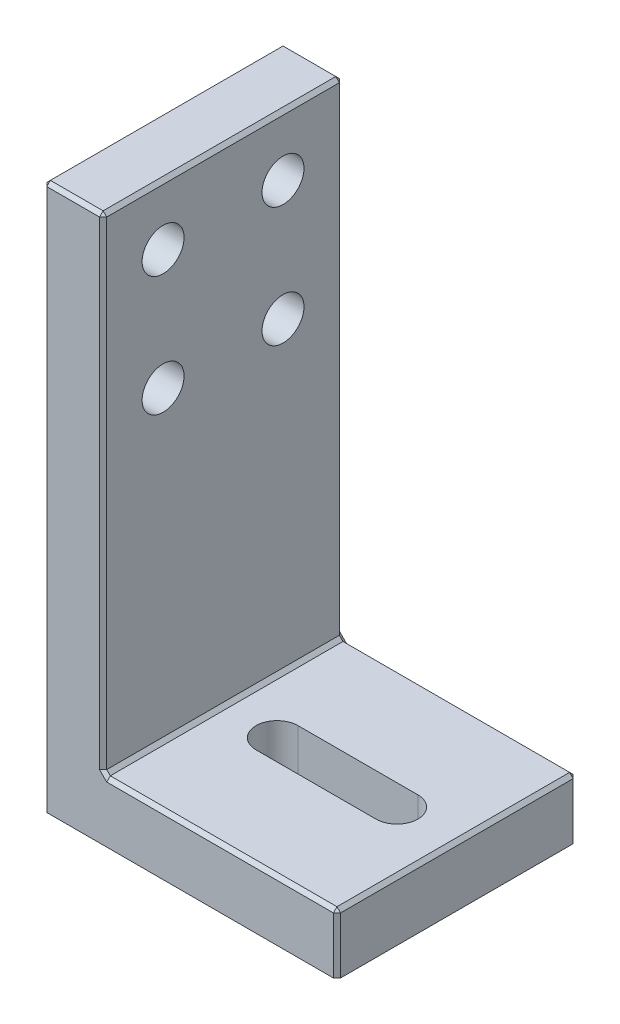
from build123d import *

# Parameters (mm, degrees)
EXTRUDE_THIN1_DEPTH = 20
CHAMFER1_SIZE       = 0.3
CUT_EXTRUDE1_REACH  = 53.386
CUT_EXTRUDE2_REACH  = 55.39
SKETCH3_R           = 1.75


with BuildPart() as part:
    # Sketch1 → Extrude-Thin1 (new body)
    with BuildSketch(Plane.XY):
        Polygon((0, 45.5), (0, 0), (24.5, 0), (24.5, 5), (5, 5), (5, 45.5), align=None)
    extrude(amount=EXTRUDE_THIN1_DEPTH)

    # Chamfer1
    chamfer1_edges = [part.edges().sort_by_distance(p)[0] for p in [
        (14.75, 5, 20),
        (5, 25.25, 20),
        (2.5, 45.5, 20),
        (0, 22.75, 20),
        (0, 22.75, 0),
        (2.5, 45.5, 0),
        (5, 25.25, 0),
        (14.75, 5, 0),
        (24.5, 2.5, 0),
        (24.5, 2.5, 20),
        (0, 0, 10),
        (0, 45.5, 10),
        (5, 45.5, 10),
        (5, 5, 10),
        (24.5, 5, 10),
    ]]
    chamfer(chamfer1_edges, length=CHAMFER1_SIZE)

    # Sketch2 → Cut-Extrude1 (cut, up to next)
    with BuildSketch(Plane(origin=(0, 5, 0), x_dir=(1, 0, 0), z_dir=(0, 1, 0)), mode=Mode.PRIVATE) as cut_extrude1_sk1:
        with BuildLine():
            Line((9.5, -8.25), (19.5, -8.25))
            ThreePointArc((19.5, -8.25), (21.25, -10), (19.5, -11.75))
            Line((19.5, -11.75), (9.5, -11.75))
            ThreePointArc((9.5, -11.75), (7.75, -10), (9.5, -8.25))
        make_face()
    cut_extrude1_tool1 = extrude(cut_extrude1_sk1.sketch, amount=-CUT_EXTRUDE1_REACH, mode=Mode.PRIVATE) & part.part
    add(cut_extrude1_tool1.solids().sort_by_distance((14.5, 5, 10))[0], mode=Mode.SUBTRACT)

    # Sketch3 → Cut-Extrude2 (cut, up to next)
    with BuildSketch(Plane(origin=(5, 0, 0), x_dir=(0, 0, -1), z_dir=(1, 0, 0)), mode=Mode.PRIVATE) as cut_extrude2_sk1:
        with Locations(Location((-15, 40.5, 0), (0, 0, 90))):
            Circle(SKETCH3_R)
    cut_extrude2_tool1 = extrude(cut_extrude2_sk1.sketch, amount=-CUT_EXTRUDE2_REACH, mode=Mode.PRIVATE) & part.part
    # Sketch3 → Cut-Extrude2 (cut, up to next)
    with BuildSketch(Plane(origin=(5, 0, 0), x_dir=(0, 0, -1), z_dir=(1, 0, 0)), mode=Mode.PRIVATE) as cut_extrude2_sk2:
        with Locations(Location((-15, 30.5, 0), (0, 0, 90))):
            Circle(SKETCH3_R)
    cut_extrude2_tool2 = extrude(cut_extrude2_sk2.sketch, amount=-CUT_EXTRUDE2_REACH, mode=Mode.PRIVATE) & part.part
    # Sketch3 → Cut-Extrude2 (cut, up to next)
    with BuildSketch(Plane(origin=(5, 0, 0), x_dir=(0, 0, -1), z_dir=(1, 0, 0)), mode=Mode.PRIVATE) as cut_extrude2_sk3:
        with Locations(Location((-5, 30.5, 0), (0, 0, 90))):
            Circle(SKETCH3_R)
    cut_extrude2_tool3 = extrude(cut_extrude2_sk3.sketch, amount=-CUT_EXTRUDE2_REACH, mode=Mode.PRIVATE) & part.part
    # Sketch3 → Cut-Extrude2 (cut, up to next)
    with BuildSketch(Plane(origin=(5, 0, 0), x_dir=(0, 0, -1), z_dir=(1, 0, 0)), mode=Mode.PRIVATE) as cut_extrude2_sk4:
        with Locations(Location((-5, 40.5, 0), (0, 0, 90))):
            Circle(SKETCH3_R)
    cut_extrude2_tool4 = extrude(cut_extrude2_sk4.sketch, amount=-CUT_EXTRUDE2_REACH, mode=Mode.PRIVATE) & part.part
    add(cut_extrude2_tool1.solids().sort_by_distance((5, 40.5, 15))[0], mode=Mode.SUBTRACT)
    add(cut_extrude2_tool2.solids().sort_by_distance((5, 30.5, 15))[0], mode=Mode.SUBTRACT)
    add(cut_extrude2_tool3.solids().sort_by_distance((5, 30.5, 5))[0], mode=Mode.SUBTRACT)
    add(cut_extrude2_tool4.solids().sort_by_distance((5, 40.5, 5))[0], mode=Mode.SUBTRACT)


solid = part.part
